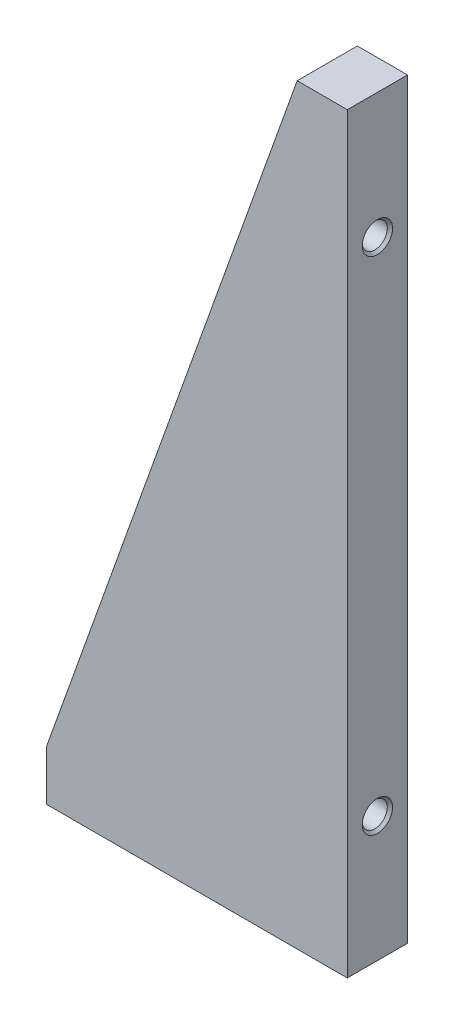
from build123d import *

# Parameters (mm, degrees)
EXTRUDE_1_DEPTH              = 12
HOLE_WIZARD_M6_1_D           = 5
HOLE_WIZARD_M6_1_DEPTH       = 15
HOLE_WIZARD_M6_1_CSINK_D     = 6.05
HOLE_WIZARD_M6_1_CSINK_ANGLE = 90
HOLE_WIZARD_M6_1_TIP         = 1.502151548
HOLE_WIZARD_M6_2_D           = 5
HOLE_WIZARD_M6_2_DEPTH       = 15
HOLE_WIZARD_M6_2_CSINK_D     = 6.05
HOLE_WIZARD_M6_2_CSINK_ANGLE = 90
HOLE_WIZARD_M6_2_TIP         = 1.502151548


with BuildPart() as part:
    # 草图1 → 凸台-拉伸1 (new body)
    with BuildSketch(Plane.XY):
        Polygon((0, 8.456375839), (0, 18.456375839), (50, 158.456375839), (60, 158.456375839), (60, 8.456375839), align=None)
    extrude(amount=EXTRUDE_1_DEPTH)

    # M6 螺纹孔1
    with Locations(Plane(origin=(0, 8.456375839, 0), x_dir=(-1, 0, 0), z_dir=(0, -1, 0))):
        with Locations((-50, -6), (-10, -6)):
            CounterSinkHole(HOLE_WIZARD_M6_1_D / 2, HOLE_WIZARD_M6_1_CSINK_D / 2, depth=HOLE_WIZARD_M6_1_DEPTH, counter_sink_angle=HOLE_WIZARD_M6_1_CSINK_ANGLE)
            with Locations((0, 0, -(HOLE_WIZARD_M6_1_DEPTH + HOLE_WIZARD_M6_1_TIP / 2))):  # 118° drill point
                Cone(0, HOLE_WIZARD_M6_1_D / 2, HOLE_WIZARD_M6_1_TIP, mode=Mode.SUBTRACT)

    # M6 螺纹孔2
    with Locations(Plane(origin=(60, 0, 0), x_dir=(0, 0, -1), z_dir=(1, 0, 0))):
        with Locations((-6, 33.456375839), (-6, 133.456375839)):
            CounterSinkHole(HOLE_WIZARD_M6_2_D / 2, HOLE_WIZARD_M6_2_CSINK_D / 2, depth=HOLE_WIZARD_M6_2_DEPTH, counter_sink_angle=HOLE_WIZARD_M6_2_CSINK_ANGLE)
            with Locations((0, 0, -(HOLE_WIZARD_M6_2_DEPTH + HOLE_WIZARD_M6_2_TIP / 2))):  # 118° drill point
                Cone(0, HOLE_WIZARD_M6_2_D / 2, HOLE_WIZARD_M6_2_TIP, mode=Mode.SUBTRACT)


solid = part.part
